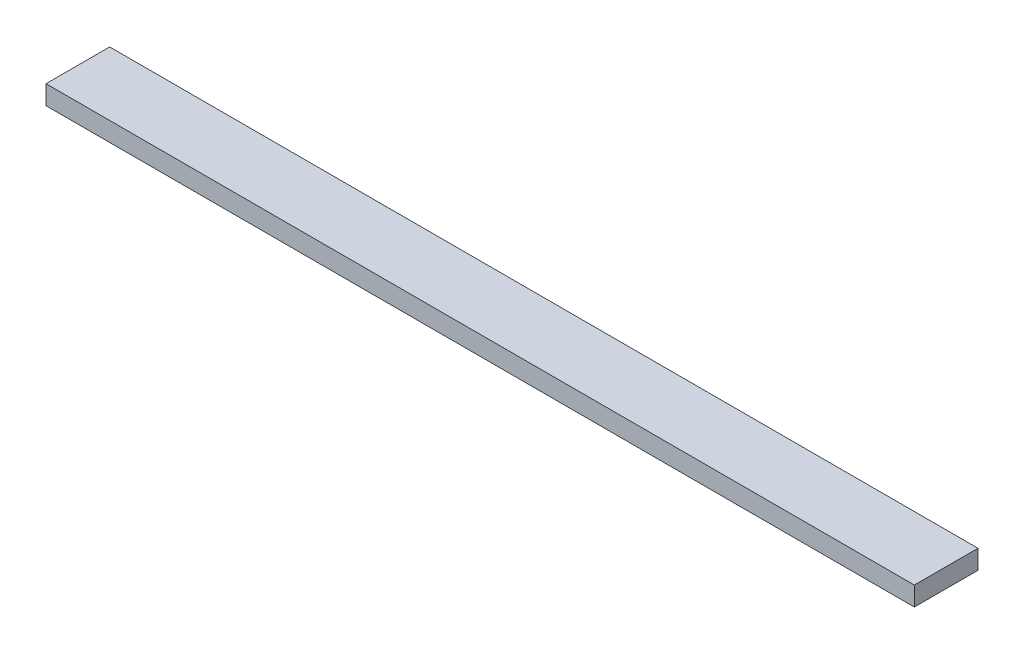
SolidWorks part; units mm, degrees
ref_plane "Front Plane" through (0, 0, 0) normal (0, 0, 1) x (1, 0, 0)
ref_plane "Top Plane" through (0, 0, 0) normal (0, 1, 0) x (1, 0, 0)
ref_plane "Right Plane" through (0, 0, 0) normal (1, 0, 0) x (0, 0, -1)
sketch "Sketch1" plane through (0, 0, 0) normal (0, 1, 0) x (1, 0, 0)
  line L1 (-682, -50) -> (682, -50)
  line L2 (-682, -50) -> (-682, 50)
  line L3 (-682, 50) -> (682, 50)
  line L4 (682, -50) -> (682, 50)
  line L5 (-682, -50) -> (682, 50) construction
  line L6 (-682, 50) -> (682, -50) construction
  point P0 (0, 0)
  dimension "D1" = 100
  dimension "D2" = 1364
extrude "Boss-Extrude1" add sketch "Sketch1" along normal blind 30
